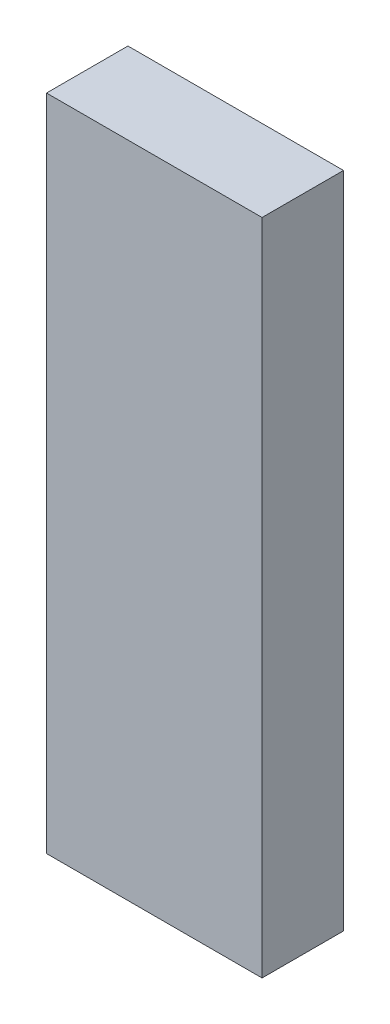
from build123d import *

# Parameters (mm, degrees)
SKETCH_1_W      = 90
SKETCH_1_H      = 275
EXTRUDE_1_DEPTH = 34


with BuildPart() as part:
    # 草图1 → 凸台-拉伸1 (new body)
    with BuildSketch(Plane.XY):
        Rectangle(SKETCH_1_W, SKETCH_1_H)
    extrude(amount=EXTRUDE_1_DEPTH)


solid = part.part
